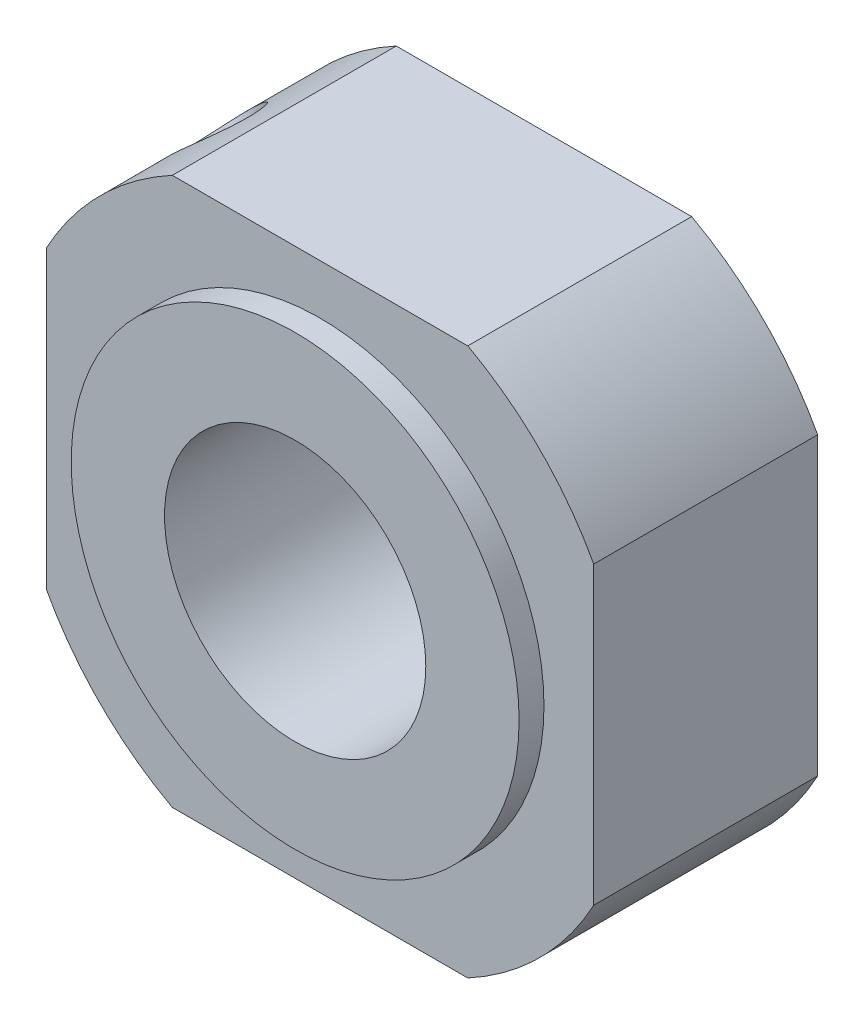
from build123d import *

# Parameters (mm, degrees)
EXTRUDE1_DEPTH             = 10
SKETCH2_OUTSIDE_W          = 30.536
SKETCH2_OUTSIDE_H          = 30.536
SKETCH2_OUTSIDE_R          = 9
EXTRUDE2_DEPTH             = 1
M4X0_7_TAPPED_HOLE1_D      = 3.3
M4X0_7_TAPPED_HOLE1_DEPTH  = 10.1
M4X0_7_TAPPED_HOLE1_TIP    = 0.991420021
M12X1_5_TAPPED_HOLE1_D     = 10.5
M12X1_5_TAPPED_HOLE1_DEPTH = 28.5
M12X1_5_TAPPED_HOLE1_TIP   = 3.15451825


with BuildPart() as part:
    # Sketch1 → Extrude1 (new body)
    with BuildSketch(Plane.XY):
        with BuildLine():
            Line((-5.937171043, -11), (5.937171043, -11))
            ThreePointArc((5.937171043, -11), (8.838834765, -8.838834765), (11, -5.937171043))
            Line((11, -5.937171043), (11, 5.937171043))
            ThreePointArc((11, 5.937171043), (8.838834765, 8.838834765), (5.937171043, 11))
            Line((5.937171043, 11), (-5.937171043, 11))
            ThreePointArc((-5.937171043, 11), (-8.838834765, 8.838834765), (-11, 5.937171043))
            Line((-11, 5.937171043), (-11, -5.937171043))
            ThreePointArc((-11, -5.937171043), (-8.838834765, -8.838834765), (-5.937171043, -11))
        make_face()
    extrude(amount=EXTRUDE1_DEPTH)

    # Sketch2 outside → Extrude2 (cut)
    with BuildSketch(Plane.XY.offset(10)):
        Rectangle(SKETCH2_OUTSIDE_W, SKETCH2_OUTSIDE_H)
        Circle(SKETCH2_OUTSIDE_R, mode=Mode.SUBTRACT)
    extrude(amount=-EXTRUDE2_DEPTH, mode=Mode.SUBTRACT)

    # M4x0.7 Tapped Hole1
    with Locations(Plane(origin=(-8.535457879, 9.132138785, 4.649594026), x_dir=(0.730571102805, 0.682836630349, 0), z_dir=(-0.682836630349, 0.730571102805, 0))):
        with Locations((0, 0)):
            Hole(M4X0_7_TAPPED_HOLE1_D / 2, depth=M4X0_7_TAPPED_HOLE1_DEPTH)
            with Locations((0, 0, -(M4X0_7_TAPPED_HOLE1_DEPTH + M4X0_7_TAPPED_HOLE1_TIP / 2))):  # 118° drill point
                Cone(0, M4X0_7_TAPPED_HOLE1_D / 2, M4X0_7_TAPPED_HOLE1_TIP, mode=Mode.SUBTRACT)

    # M12x1.5 Tapped Hole1
    with Locations(Plane.XY.offset(10)):
        with Locations((0, 0)):
            Hole(M12X1_5_TAPPED_HOLE1_D / 2, depth=M12X1_5_TAPPED_HOLE1_DEPTH)
            with Locations((0, 0, -(M12X1_5_TAPPED_HOLE1_DEPTH + M12X1_5_TAPPED_HOLE1_TIP / 2))):  # 118° drill point
                Cone(0, M12X1_5_TAPPED_HOLE1_D / 2, M12X1_5_TAPPED_HOLE1_TIP, mode=Mode.SUBTRACT)


solid = part.part
